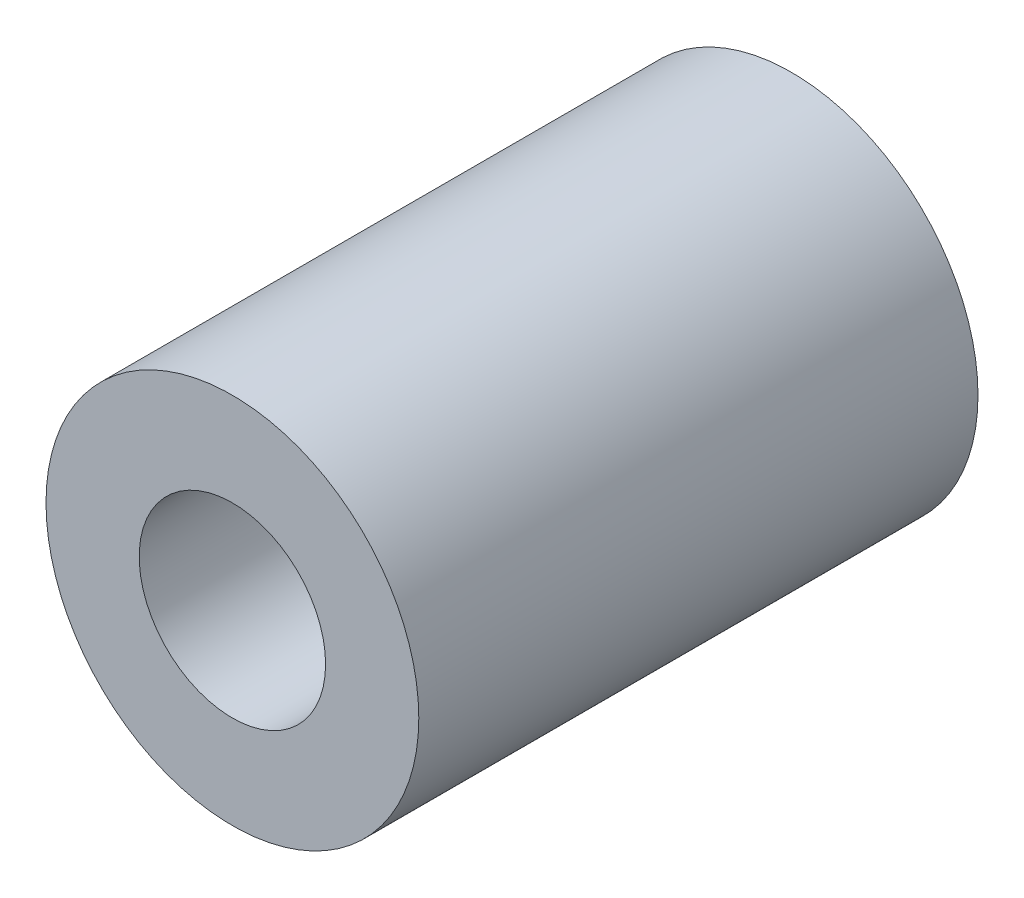
from build123d import *

# Parameters (mm, degrees)
SKETCH_1_R                = 10
EXTRUDE_1_DEPTH           = 15
HOLE_WIZARD_1_D           = 5.5
HOLE_WIZARD_1_CBORE_D     = 10
HOLE_WIZARD_1_CBORE_DEPTH = 12


with BuildPart() as part:
    # 草图1 → 凸台-拉伸1 (new, symmetric)
    with BuildSketch(Plane.XY):
        Circle(SKETCH_1_R)
    extrude(amount=EXTRUDE_1_DEPTH, both=True)

    # 打孔尺寸(%根据)内六角圆柱头螺钉的类型1 (through all)
    with Locations(Plane.XY.offset(15)):
        with Locations((0, 0)):
            CounterBoreHole(HOLE_WIZARD_1_D / 2, HOLE_WIZARD_1_CBORE_D / 2, HOLE_WIZARD_1_CBORE_DEPTH)


solid = part.part
